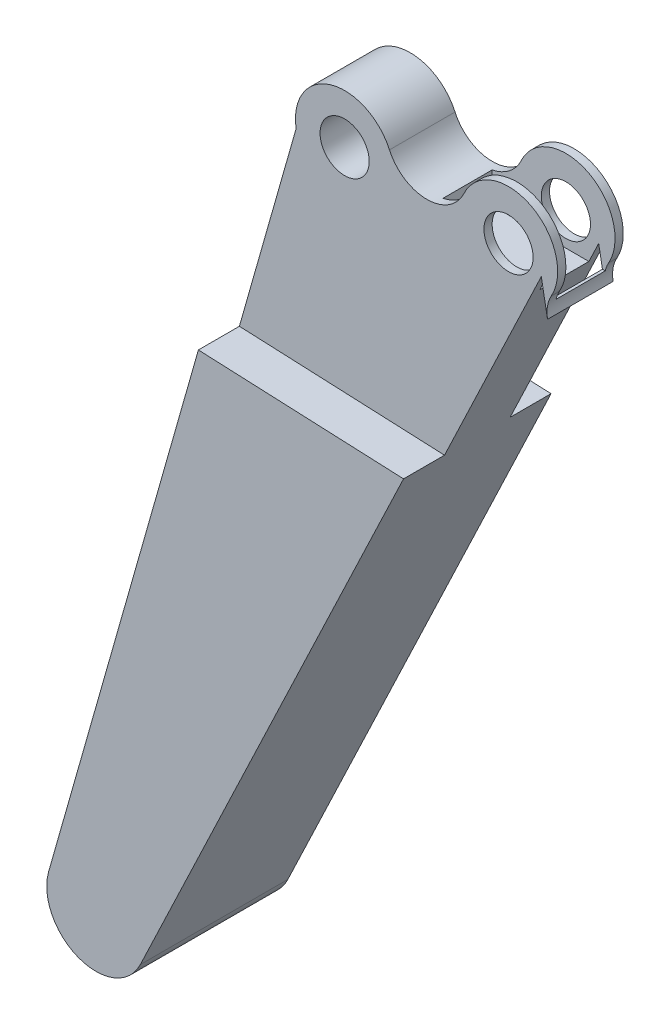
SolidWorks part; units mm, degrees
material "1060 Alloy"
ref_plane "Front Plane" through (0, 0, 0) normal (0, 0, 1) x (1, 0, 0)
ref_plane "Top Plane" through (0, 0, 0) normal (0, 1, 0) x (1, 0, 0)
ref_plane "Right Plane" through (0, 0, 0) normal (1, 0, 0) x (0, 0, -1)
sketch "Sketch1" plane through (0, 0, 0) normal (0, 0, 1) x (1, 0, 0)
  line L2 (-3.5906, -11.6394) -> (-4.3454, -7.4963)
  line L3 (-4.3454, -7.4963) -> (-48.2794, -99.6762)
  line L5 (-59.4669, -95.4537) -> (-34.2653, -6.8245)
  circle A0 centre (-28.3474, -5.8356) radius 3
  circle A1 centre (-8.3479, -5.9788) radius 3
  arc A2 (-22.8751, -3.3751) -> (-34.2653, -6.8245) centre (-28.3474, -5.8356) ccw
  arc A3 (-3.1324, -8.945) -> (-13.7844, -3.4402) centre (-8.3479, -5.9788) ccw
  arc A4 (-22.8751, -3.3751) -> (-13.7844, -3.4402) centre (-18.3148, -1.3247) ccw
  arc A5 (-3.5906, -11.6394) -> (-3.1324, -8.945) centre (0.3446, -10.9225) cw
  arc A6 (-59.4669, -95.4537) -> (-48.2794, -99.6762) centre (-53.6956, -97.0947) ccw
  dimension "D1" = 6
  dimension "D2" = 6
  dimension "D4" = 12
  dimension "D5" = 12
  dimension "D6" = 10
  dimension "D7" = 4
  dimension "D8" = 6
  dimension "D3" = 20
extrude "Boss-Extrude1" add sketch "Sketch1" along normal blind 8 contours L5 A6 L3 L2 A5 A3 A4 A2 A0 A1
sketch "Sketch2" plane through (0, 0, 0) normal (0, 1, 0) x (1, 0, 0)
  line L0 (-2.3479, -8) -> (-2.3479, 0) construction
  line L1 (12.6521, -1) -> (-17.3479, -1)
  line L2 (12.6521, -1) -> (12.6521, -7)
  line L3 (12.6521, -7) -> (-17.3479, -7)
  line L4 (-17.3479, -1) -> (-17.3479, -7)
  line L5 (12.6521, -1) -> (-17.3479, -7) construction
  line L6 (12.6521, -7) -> (-17.3479, -1) construction
  point P0 (-2.3479, -4)
  dimension "D1" = 6
  dimension "D2" = 30
extrude "Cut-Extrude1" cut sketch "Sketch2" against normal blind 10 and the other way blind 10
sketch "Sketch3" plane through (0, 0, 8) normal (0, 0, 1) x (1, 0, 0)
  line L0 (-16.1584, -32.2816) -> (-41.189, -31.1738)
  line L1 (-4.3454, -7.4963) -> (-48.2794, -99.6762) construction
  line L2 (-59.4669, -95.4537) -> (-34.2653, -6.8245) construction
  line L3 (-41.189, -31.1738) -> (-59.4669, -95.4537)
  line L5 (-48.2794, -99.6762) -> (-16.1584, -32.2816)
  arc A0 (-59.4669, -95.4537) -> (-48.2794, -99.6762) centre (-53.6956, -97.0947) ccw
  arc A1 (-59.4669, -95.4537) -> (-48.2794, -99.6762) centre (-53.6956, -97.0947) ccw construction
extrude "Boss-Extrude2" add sketch "Sketch3" along normal blind 5
ref_plane "Plane1" through (0, 0, 4) normal (0, 0, 1) x (1, 0, 0)
mirror "Mirror1" about plane through (0, 0, 4) normal (0, 0, 1) of "Boss-Extrude2"
scale "Scale1" scale about origin uniform scaling yes scale factor 0.5
